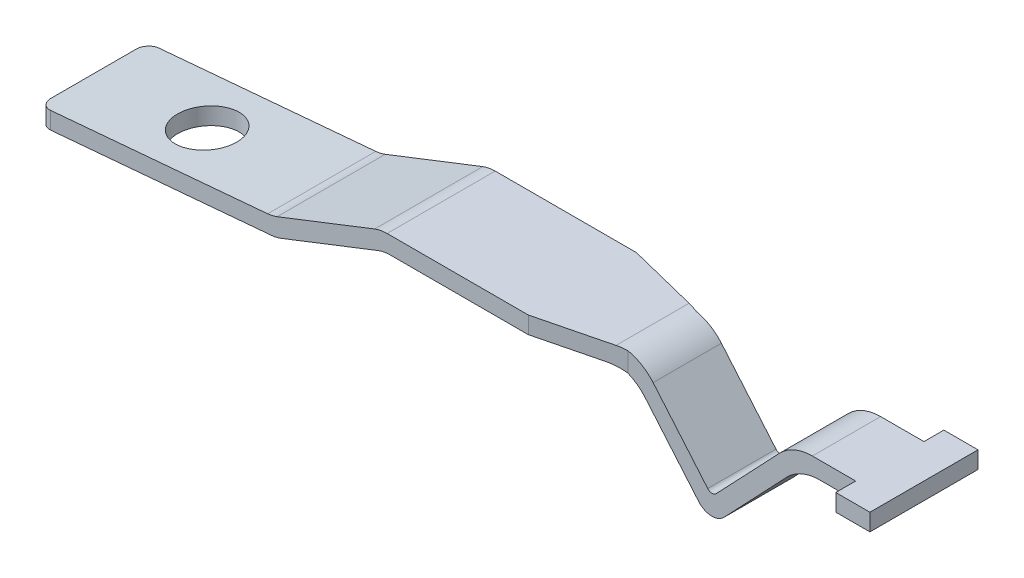
from build123d import *

# Parameters (mm, degrees)
BOSS_EXTRUDE1_DEPTH = 4.75
SKETCH2_OUTSIDE_W   = 89.832
SKETCH2_OUTSIDE_H   = 26.332
SKETCH2_OUTSIDE_R   = 2.6
CUT_EXTRUDE1_DEPTH  = 30


with BuildPart() as part:
    # Sketch1 → Boss-Extrude1 (new, symmetric)
    with BuildSketch(Plane.XY):
        with BuildLine():
            Line((128.472093399, 20.626012941), (135.279511004, 20.626012941))
            Line((135.279511004, 20.626012941), (135.279511004, 19.126012941))
            Line((135.279511004, 19.126012941), (129.116456396, 19.126012941))
            ThreePointArc((129.116456396, 19.126012941), (127.537662704, 18.801255856), (126.215231232, 17.879718181))
            Line((126.215231232, 17.879718181), (120.723107444, 12.093373476))
            ThreePointArc((120.723107444, 12.093373476), (119.592910743, 11.626607721), (118.490782391, 12.156256613))
            Line((118.490782391, 12.156256613), (113.782718692, 17.712029816))
            ThreePointArc((113.782718692, 17.712029816), (112.412732854, 18.755342597), (110.731077047, 19.126012941))
            Line((110.731077047, 19.126012941), (93.127493614, 19.126012941))
            ThreePointArc((93.127493614, 19.126012941), (92.571949476, 19.074126018), (92.035622322, 18.920260082))
            Line((92.035622322, 18.920260082), (83.526071058, 15.595094388))
            ThreePointArc((83.526071058, 15.595094388), (83.117810035, 15.468266897), (82.695666994, 15.400757434))
            Line((82.695666994, 15.400757434), (62.410244618, 13.626012941))
            Line((62.410244618, 13.626012941), (62.279511004, 15.120304988))
            Line((62.279511004, 15.120304988), (82.350355756, 16.876276372))
            ThreePointArc((82.350355756, 16.876276372), (82.772498797, 16.943785835), (83.180759819, 17.070613325))
            Line((83.180759819, 17.070613325), (91.752961452, 20.420260082))
            ThreePointArc((91.752961452, 20.420260082), (92.289288606, 20.574126018), (92.844832744, 20.626012941))
            Line((92.844832744, 20.626012941), (111.42610449, 20.626012941))
            ThreePointArc((111.42610449, 20.626012941), (113.107760296, 20.255342597), (114.477746134, 19.212029816))
            Line((114.477746134, 19.212029816), (119.274777803, 13.551269534))
            ThreePointArc((119.274777803, 13.551269534), (119.64215392, 13.374719903), (120.018886154, 13.530308488))
            Line((120.018886154, 13.530308488), (125.570868236, 19.379718181))
            ThreePointArc((125.570868236, 19.379718181), (126.893299708, 20.301255856), (128.472093399, 20.626012941))
        make_face()
    extrude(amount=BOSS_EXTRUDE1_DEPTH, both=True)

    # Sketch2 outside → Cut-Extrude1 (cut)
    # profile 1 of 2: a face of its own
    with BuildSketch(Plane(origin=(0, 0, 0), x_dir=(1, 0, 0), z_dir=(0, 1, 0))):
        with Locations((98.78, 0)):
            Rectangle(SKETCH2_OUTSIDE_W, SKETCH2_OUTSIDE_H)
        with BuildLine():
            Line((132.279511004, 4.75), (132.279511004, 3))
            Line((132.279511004, 3), (112.256897869, 3))
            Line((112.256897869, 3), (105.256897869, 4.75))
            Line((105.256897869, 4.75), (63.279511004, 4.75))
            ThreePointArc((63.279511004, 4.75), (62.572404223, 4.457106781), (62.279511004, 3.75))
            Line((62.279511004, 3.75), (62.279511004, -3.75))
            ThreePointArc((62.279511004, -3.75), (62.572404223, -4.457106781), (63.279511004, -4.75))
            Line((63.279511004, -4.75), (105.256897869, -4.75))
            Line((105.256897869, -4.75), (112.256897869, -3))
            Line((112.256897869, -3), (132.279511004, -3))
            Line((132.279511004, -3), (132.279511004, -4.75))
            Line((132.279511004, -4.75), (135.279511004, -4.75))
            Line((135.279511004, -4.75), (135.279511004, 4.75))
            Line((135.279511004, 4.75), (132.279511004, 4.75))
        make_face(mode=Mode.SUBTRACT)
    # profile 2 of 2: a face of its own
    with BuildSketch(Plane(origin=(0, 0, 0), x_dir=(1, 0, 0), z_dir=(0, 1, 0))):
        with Locations(Location((72.279511004, 0, 0), (0, 0, 180))):
            Circle(SKETCH2_OUTSIDE_R)
    extrude(amount=CUT_EXTRUDE1_DEPTH, mode=Mode.SUBTRACT)


solid = part.part
